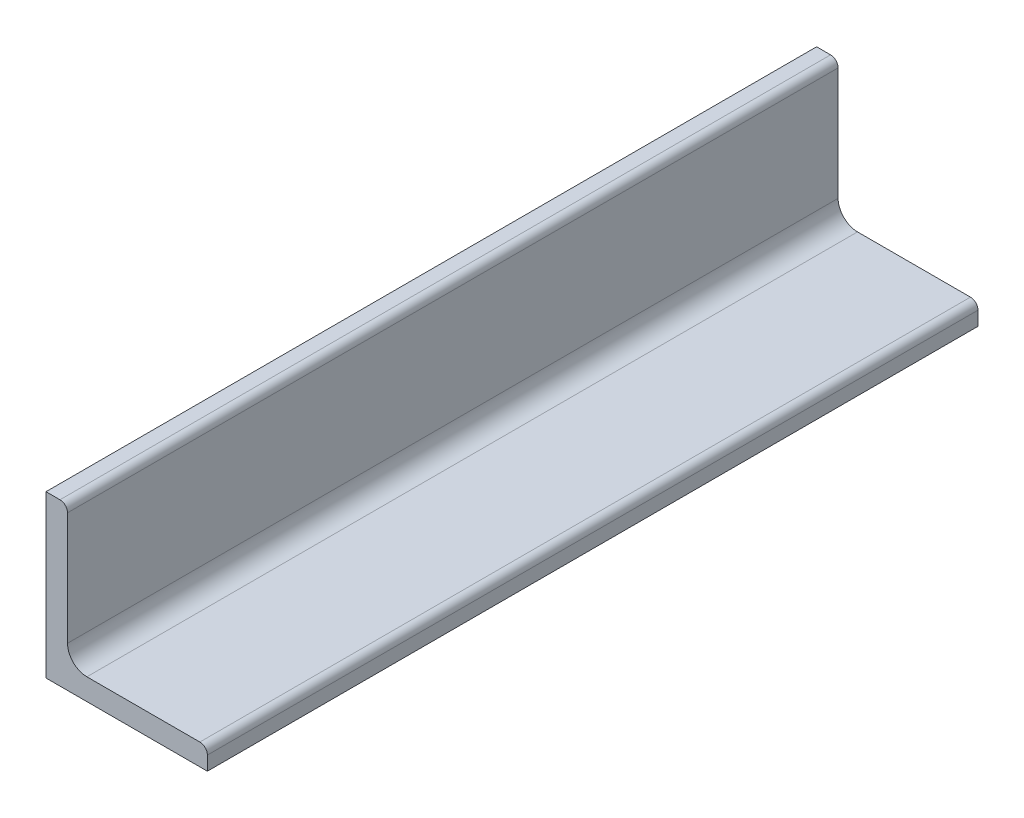
from build123d import *

# Parameters (mm, degrees)
BOSS_EXTRUDE1_DEPTH = 179.05


with BuildPart() as part:
    # Sketch1 → Boss-Extrude1 (new, symmetric)
    with BuildSketch(Plane.XY):
        with BuildLine():
            Line((0, 75), (0, 0))
            Line((0, 0), (75, 0))
            Line((75, 0), (75, 6.5))
            ThreePointArc((75, 6.5), (73.974873734, 8.974873734), (71.5, 10))
            Line((71.5, 10), (19, 10))
            ThreePointArc((19, 10), (12.636038969, 12.636038969), (10, 19))
            Line((10, 19), (10, 71.5))
            ThreePointArc((10, 71.5), (8.974873734, 73.974873734), (6.5, 75))
            Line((6.5, 75), (0, 75))
        make_face()
    extrude(amount=BOSS_EXTRUDE1_DEPTH, both=True)


solid = part.part
